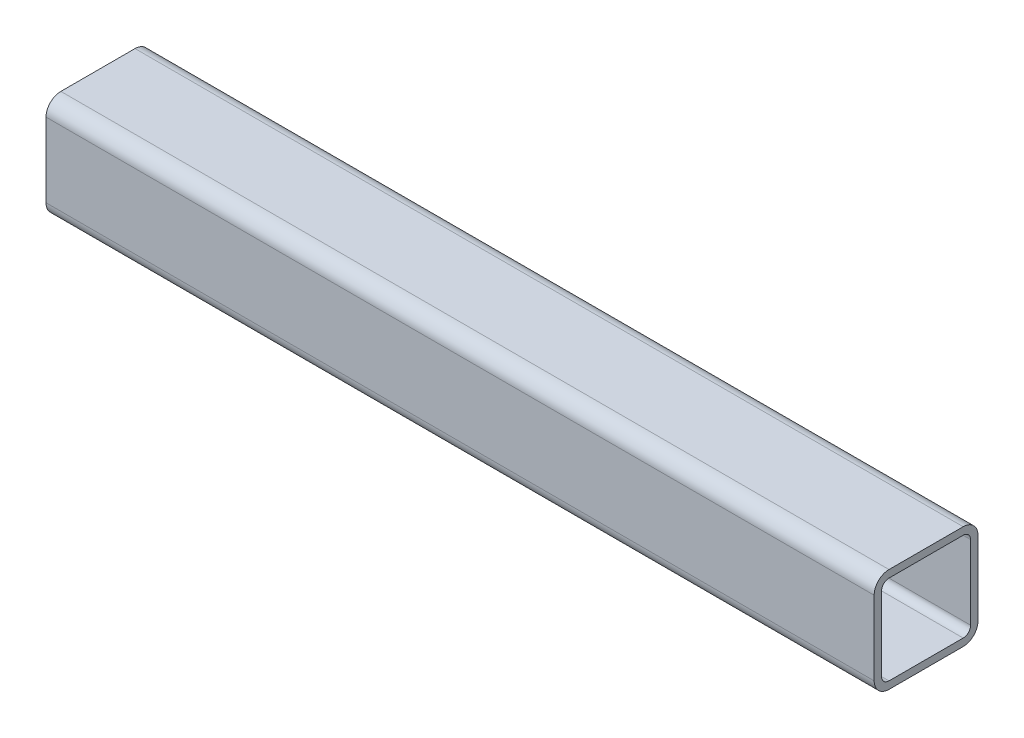
SolidWorks part; units mm, degrees
ref_plane "Front Plane" through (0, 0, 0) normal (0, 0, 1) x (1, 0, 0)
ref_plane "Top Plane" through (0, 0, 0) normal (0, 1, 0) x (1, 0, 0)
ref_plane "Right Plane" through (0, 0, 0) normal (1, 0, 0) x (0, 0, -1)
ref_plane "Plane4" through (249, 0, 0) normal (1, 0, 0) x (0, 0, -1)
sketch "Sketch1" plane through (249, 0, 0) normal (1, 0, 0) x (0, 0, -1)
  line L0 (40, -28.5714) -> (40, 28.5714)
  line L1 (28.5714, 40) -> (-28.5714, 40)
  line L2 (-40, 28.5714) -> (-40, -28.5714)
  line L3 (-28.5714, -40) -> (28.5714, -40)
  line L4 (-34.2857, -28.5714) -> (-34.2857, 28.5714)
  line L5 (-28.5714, 34.2857) -> (28.5714, 34.2857)
  line L6 (34.2857, 28.5714) -> (34.2857, -28.5714)
  line L7 (28.5714, -34.2857) -> (-28.5714, -34.2857)
  arc A0 (28.5714, -40) -> (40, -28.5714) centre (28.5714, -28.5714) ccw
  arc A1 (40, 28.5714) -> (28.5714, 40) centre (28.5714, 28.5714) ccw
  arc A2 (-28.5714, 40) -> (-40, 28.5714) centre (-28.5714, 28.5714) ccw
  arc A3 (-40, -28.5714) -> (-28.5714, -40) centre (-28.5714, -28.5714) ccw
  arc A4 (-28.5714, -34.2857) -> (-34.2857, -28.5714) centre (-28.5714, -28.5714) cw
  arc A5 (-34.2857, 28.5714) -> (-28.5714, 34.2857) centre (-28.5714, 28.5714) cw
  arc A6 (28.5714, 34.2857) -> (34.2857, 28.5714) centre (28.5714, 28.5714) cw
  arc A7 (34.2857, -28.5714) -> (28.5714, -34.2857) centre (28.5714, -28.5714) cw
  dimension "D1" = 80
  dimension "D2" = 57.1429
extrude "Boss-Extrude1" add sketch "Sketch1" against normal blind 638
